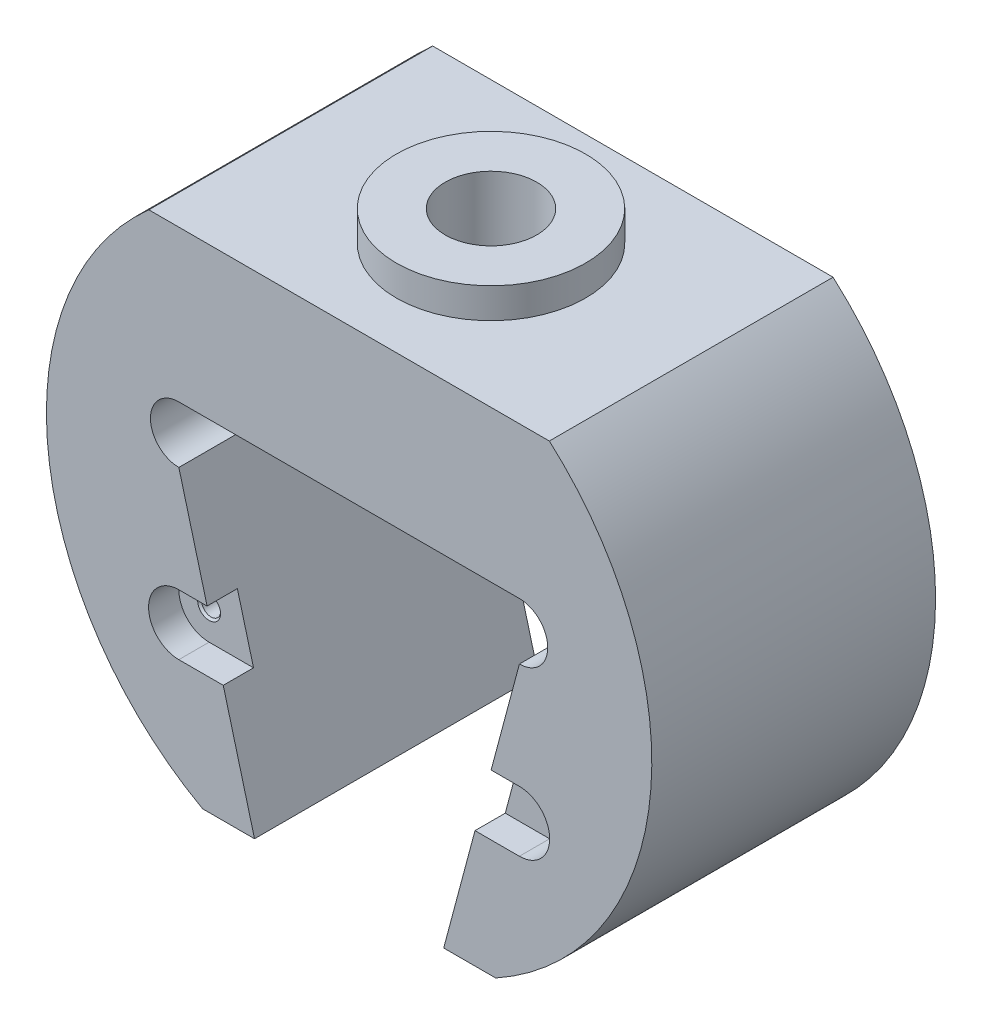
SolidWorks part; units mm, degrees
ref_plane "Front Plane" through (0, 0, 0) normal (0, 0, 1) x (1, 0, 0)
ref_plane "Top Plane" through (0, 0, 0) normal (0, 1, 0) x (1, 0, 0)
ref_plane "Right Plane" through (0, 0, 0) normal (1, 0, 0) x (0, 0, -1)
other "Configuration Table"
sketch "Sketch1" plane through (0, 0, 0) normal (0, 0, 1) x (1, 0, 0)
  circle A0 centre (0, 0) radius 80
  dimension "D1" = 160
extrude "Boss-Extrude1" add sketch "Sketch1" along normal blind 75
sketch "Sketch2" plane through (0, 0, 0) normal (0, 0, -1) x (-1, 0, 0)
  line L1 (-98.8631, 60) -> (100.7807, 60)
  line L2 (-98.8631, 60) -> (-98.8631, -70)
  line L3 (-98.8631, -70) -> (100.7807, -70)
  line L4 (100.7807, 60) -> (100.7807, -70)
  circle A0 centre (0, 0) radius 80 construction
  dimension "D1" = 130
  dimension "D2" = 199.6438
  dimension "D3" = 70
extrude "Cut-Extrude1" cut sketch "Sketch2" against normal through all flip side to cut
sketch "Sketch3" plane through (0, 0, 0) normal (0, 0, -1) x (-1, 0, 0)
  line L0 (0, 60) -> (0, -75.8048) construction
  line L1 (-52.915, 60) -> (52.915, 60) construction
  line L2 (-25, -70) -> (-45, 5)
  line L3 (38.7298, -70) -> (-38.7298, -70) construction
  line L4 (-45, 20) -> (45, 20)
  line L5 (25, -70) -> (45, 5)
  line L6 (-25, -70) -> (25, -70)
  arc A0 (-45, 20) -> (-45, 5) centre (-45, 12.5) ccw
  arc A1 (45, 20) -> (45, 5) centre (45, 12.5) cw
  point P11 (0, 20)
  dimension "D4" = 15
  dimension "D1" = 90
  dimension "D2" = 45
  dimension "D3" = 25
  dimension "D5" = 45
extrude "Cut-Extrude2" cut sketch "Sketch3" against normal through all
sketch "Sketch4" plane through (0, 0, 0) normal (0, 0, -1) x (-1, 0, 0)
  line L0 (-45, -31) -> (45, -31) construction
  line L1 (-45, -23) -> (45, -23)
  line L2 (-45, -39) -> (45, -39)
  line L3 (-25, -70) -> (-38.7298, -70) construction
  arc A0 (-45, -23) -> (-45, -39) centre (-45, -31) ccw
  arc A1 (45, -39) -> (45, -23) centre (45, -31) ccw
  point P2 (0, -31)
  dimension "D1" = 8
  dimension "D2" = 39
  dimension "D3" = 45
  dimension "D4" = 90
extrude "Cut-Extrude3" cut sketch "Sketch4" against normal blind 8
sketch "Sketch5" plane through (0, 0, 8) normal (0, 0, -1) x (-1, 0, 0)
  line L0 (37.5333, -23) -> (33.2667, -39) construction
  line L1 (33.2667, -39) -> (45, -39) construction
  line L2 (45, -23) -> (37.5333, -23) construction
  line L3 (-33.2667, -39) -> (-37.5333, -23) construction
  line L4 (-37.5333, -23) -> (-45, -23) construction
  line L5 (-45, -39) -> (-33.2667, -39) construction
  line L6 (37.5333, -23) -> (33.2667, -39)
  line L7 (33.2667, -39) -> (45, -39)
  line L8 (45, -23) -> (37.5333, -23)
  line L9 (-33.2667, -39) -> (-37.5333, -23)
  line L10 (-37.5333, -23) -> (-45, -23)
  line L11 (-45, -39) -> (-33.2667, -39)
  arc A0 (45, -39) -> (45, -23) centre (45, -31) ccw construction
  arc A1 (-45, -23) -> (-45, -39) centre (-45, -31) ccw construction
  arc A2 (45, -39) -> (45, -23) centre (45, -31) ccw
  arc A3 (-45, -23) -> (-45, -39) centre (-45, -31) ccw
extrude "Cut-Extrude4" cut sketch "Sketch5" against normal blind 8 from offset 59 offset against normal yes
hole_wizard "M6 Tapped Hole1" positions "3DSketch1" profile "Sketch6" tap size "M6" standard "GB"
sketch3d "3DSketch1"
  line L0 (45, -31, 8) -> (45, -31, 0) construction
  line L1 (-45, -31, 8) -> (-45, -31, 0) construction
  line L2 (-45, -31, 75) -> (-45, -31, 67) construction
  line L3 (45, -31, 75) -> (45, -31, 67) construction
  point P0 (45, -31, 8)
  point P4 (-45, -31, 8)
  point P8 (-45, -31, 67)
  point P12 (45, -31, 67)
sketch "Sketch6" plane through (45, -31, 8) normal (1, 0, 0) x (0, 1, 0)
  line L0 (0, 0) -> (0, 16.5022)
  line L1 (0, 16.5022) -> (2.5, 15)
  line L2 (2.5, 15) -> (2.5, 0.525)
  line L3 (2.5, 0.525) -> (3.025, 0)
  line L5 (3.025, 0) -> (0, 0)
  line L6 (-2.5, 0.525) -> (-3.025, 0) construction
  line L10 (0, 16.5022) -> (-2.5, 15) construction
  line L11 (0, -6.35) -> (0, 107.95) construction
  dimension "螺纹孔钻头直径" = 5
  dimension "螺纹孔钻头深度" = 15
  dimension "近端锥形沉头孔直径" = 6.05
  dimension "近端锥形沉头孔角度" = 90
  dimension "导头角度" = 118
cosmetic thread "Hole Thread1" parameters "D1"=12, "D2"=6
cosmetic thread "Hole Thread2" parameters "D1"=12, "D2"=6
cosmetic thread "Hole Thread3" parameters "D1"=12, "D2"=6
cosmetic thread "Hole Thread4" parameters "D1"=12, "D2"=6
sketch "Sketch7" plane through (0, 60, 0) normal (0, 1, 0) x (1, 0, 0)
  line L0 (-52.915, -37.5) -> (52.915, -37.5) construction
  line L1 (-52.915, 0) -> (-52.915, -75) construction
  line L2 (52.915, -75) -> (52.915, 0) construction
  line L3 (0, 0) -> (0, -75) construction
  line L4 (-52.915, -75) -> (52.915, -75) construction
  circle A0 centre (0, -37.5) radius 12.1
  dimension "D1" = 24.2
extrude "Cut-Extrude5" cut sketch "Sketch7" against normal up to next
sketch "Sketch8" plane through (0, 60, 0) normal (0, 1, 0) x (1, 0, 0)
  circle A0 centre (0, -37.5) radius 25
  circle A1 centre (0, -37.5) radius 12.1
  dimension "D1" = 50
extrude "Boss-Extrude4" add sketch "Sketch8" along normal blind 8
